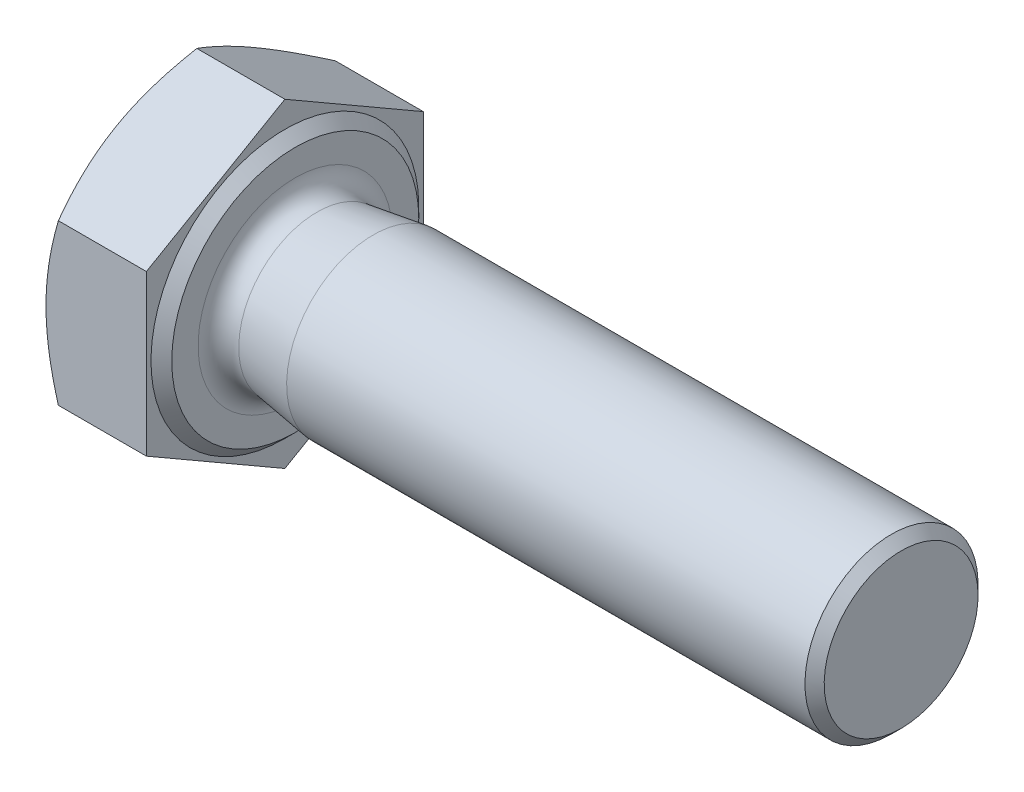
from build123d import *

# Parameters (mm, degrees)
EXTRUDE_1_DEPTH     = 6.4
SKETCH_4_R          = 17.59
SKETCH_4_R_2        = 8
CUT_EXTRUDE_1_DEPTH = 0.8
CUT_EXTRUDE_1_DRAFT = -60
CHAMFER_1_SIZE      = 0.555555556


with BuildPart() as part:
    # 草图3 → 凸台-拉伸1 (new body)
    with BuildSketch(Plane(origin=(0, 0, 0), x_dir=(0, 0, -1), z_dir=(1, 0, 0))):
        Polygon((8, 4.618802154), (0, 9.237604307), (-8, 4.618802154), (-8, -4.618802154), (0, -9.237604307), (8, -4.618802154), align=None)
    extrude(amount=EXTRUDE_1_DEPTH)


with BuildPart() as cut_extrude_1_tool:
    # 草图4 → 切除-拉伸1 (with draft: the straight prism first)
    with BuildSketch(Plane.ZY):
        Circle(SKETCH_4_R)
        Circle(SKETCH_4_R_2, mode=Mode.SUBTRACT)
    extrude(amount=-CUT_EXTRUDE_1_DEPTH)
    # 切除-拉伸1: the draft: its side faces are tilted about the plane it starts from
    cut_extrude_1_sides = [cut_extrude_1_tool.faces().sort_by_distance(p)[0] for p in [
        (0.4, 0, -17.59),
        (0.4, 0, -8),
    ]]
    draft(cut_extrude_1_sides, Plane.ZY, CUT_EXTRUDE_1_DRAFT)


with BuildPart() as part_1:
    add(part.part)

    # 切除-拉伸1: cut by cut_extrude_1_tool
    add(cut_extrude_1_tool.part, mode=Mode.SUBTRACT)

    # 草图6 → 旋转2 (revolve)
    with BuildSketch(Plane.XY, mode=Mode.PRIVATE) as revolve_2_sk:
        with BuildLine():
            Line((10.9, 5), (41.4, 5))
            Line((41.4, 5), (41.4, 0))
            Line((41.4, 0), (6.4, 0))
            Line((6.4, 0), (6.4, 5.612875))
            ThreePointArc((6.4, 5.612875), (6.78085818, 4.780507868), (7.659700078, 4.524529519))
            Line((7.659700078, 4.524529519), (10.9, 5))
        make_face()
    revolve(revolve_2_sk.sketch.rotate(Axis((6.4, 0, 0), (1, 0, 0)), 180), axis=Axis((6.4, 0, 0), (1, 0, 0)))

    # 倒角1
    chamfer_1_edges = [part_1.edges().sort_by_distance(p)[0] for p in [
        (41.4, 5, 0),
    ]]
    chamfer(chamfer_1_edges, length=CHAMFER_1_SIZE)

    # 草图8 → 切除-旋转2 (revolve, cut)
    with BuildSketch(Plane.XY, mode=Mode.PRIVATE) as cut_revolve_2_sk:
        Polygon((6.4, 7.135), (5.8, 7.735), (5.8, 17.59), (6.4, 17.59), align=None)
    revolve(cut_revolve_2_sk.sketch.rotate(Axis((0, 0, 0), (1, 0, 0)), 180), axis=Axis((0, 0, 0), (1, 0, 0)), mode=Mode.SUBTRACT)


solid = part_1.part
